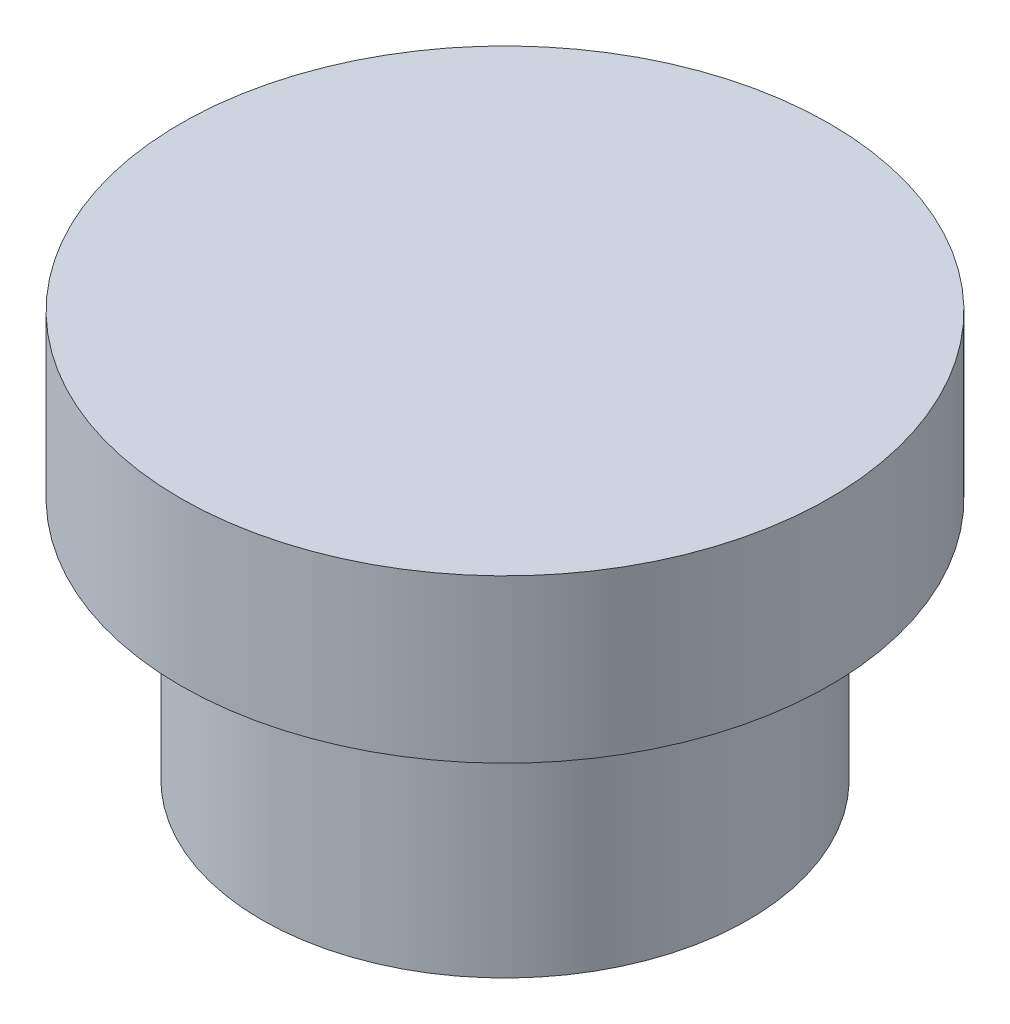
SolidWorks part; units mm, degrees
ref_plane "Front Plane" through (0, 0, 0) normal (0, 0, 1) x (1, 0, 0)
ref_plane "Top Plane" through (0, 0, 0) normal (0, 1, 0) x (1, 0, 0)
ref_plane "Right Plane" through (0, 0, 0) normal (1, 0, 0) x (0, 0, -1)
other "Configuration Table"
sketch "Sketch1" plane through (0, 0, 0) normal (0, 0, 1) x (1, 0, 0)
  line L0 (0, 0) -> (4, 0)
  line L1 (4, 0) -> (4, -2)
  line L2 (4, -2) -> (3, -2)
  line L3 (3, -2) -> (3, -5)
  line L4 (3, -5) -> (0, -5)
  line L5 (0, -5) -> (0, 0)
  dimension "D1" = 3
  dimension "D2" = 4
  dimension "D3" = 2
  dimension "D4" = 5
revolve "Revolve1" add sketch "Sketch1" angle 360 about L5
